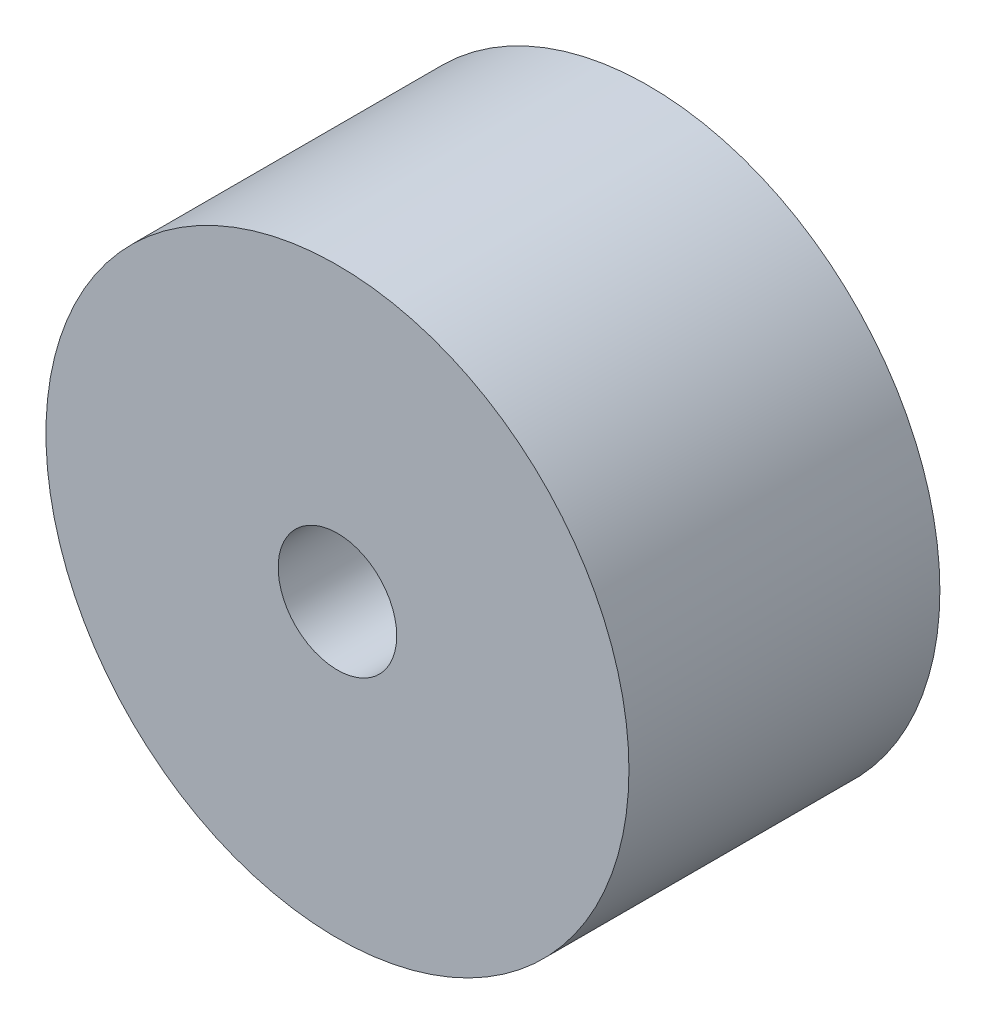
from build123d import *

# Parameters (mm, degrees)
SKETCH_1_R      = 30
SKETCH_1_R_2    = 6.1
EXTRUDE_1_DEPTH = 16


with BuildPart() as part:
    # 草图1 → 凸台-拉伸1 (new, symmetric)
    with BuildSketch(Plane.XY):
        Circle(SKETCH_1_R)
        Circle(SKETCH_1_R_2, mode=Mode.SUBTRACT)
    extrude(amount=EXTRUDE_1_DEPTH, both=True)


solid = part.part
